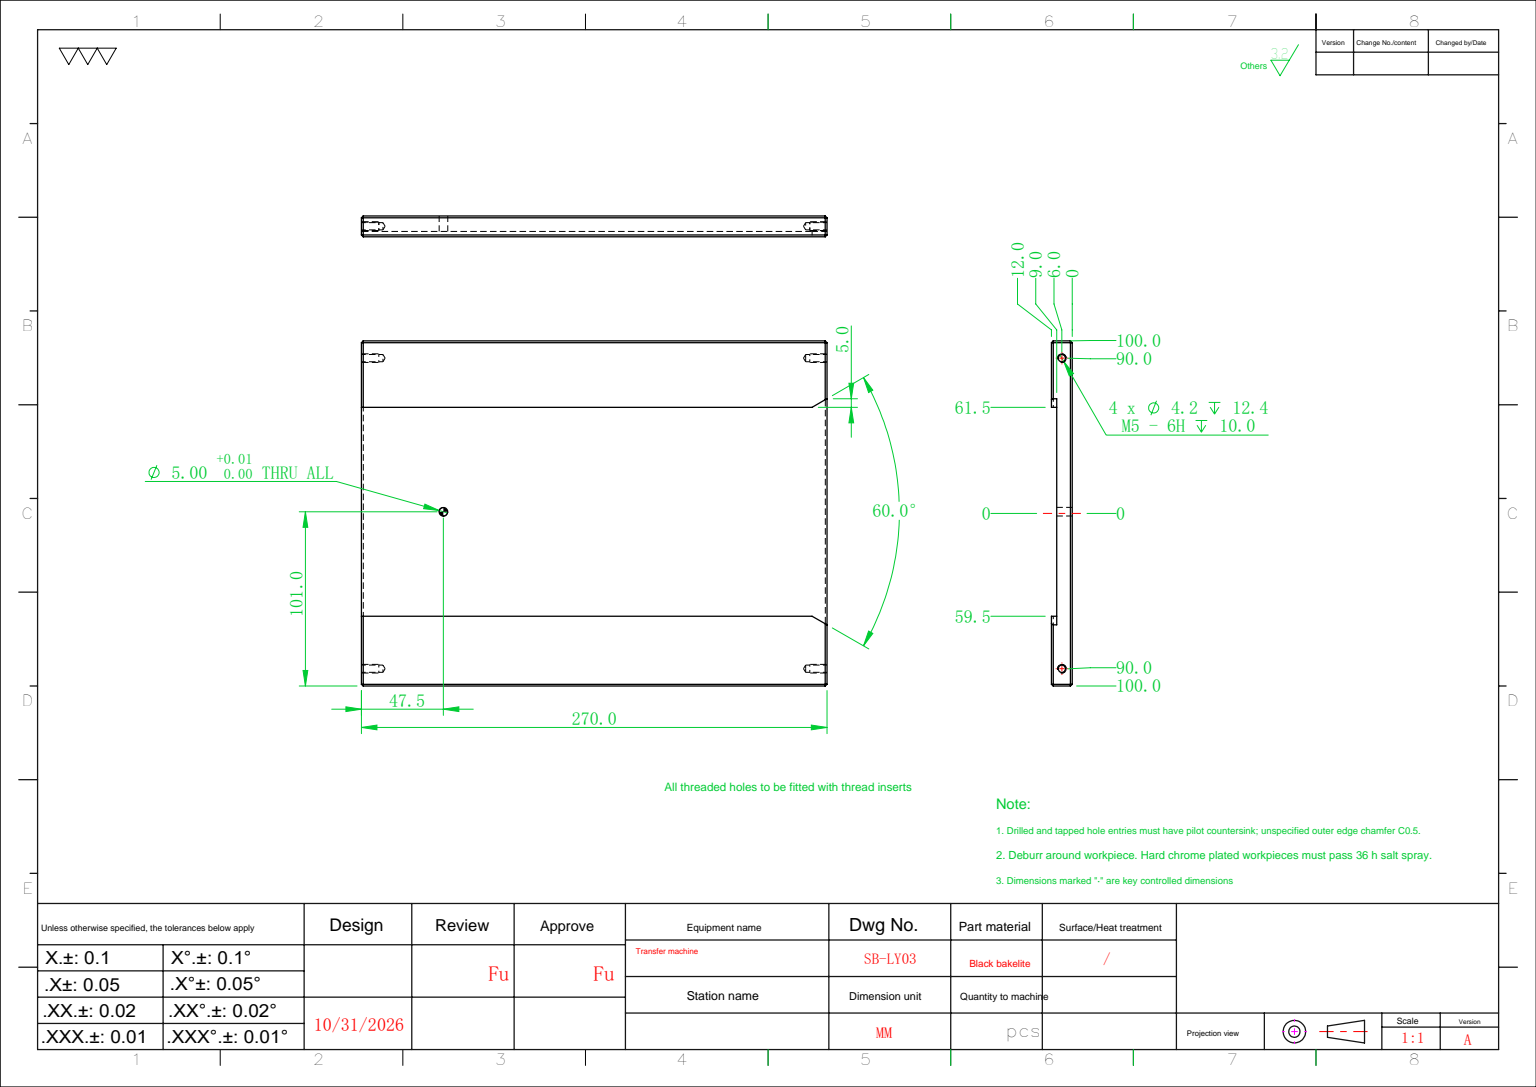
SolidWorks part; units mm, degrees
ref_plane "前视基准面" through (0, 0, 0) normal (0, 0, 1) x (1, 0, 0)
ref_plane "上视基准面" through (0, 0, 0) normal (0, 1, 0) x (1, 0, 0)
ref_plane "右视基准面" through (0, 0, 0) normal (1, 0, 0) x (0, 0, -1)
sketch "草图1" plane through (0, 0, 0) normal (0, 0, 1) x (1, 0, 0)
  line L1 (-100, -135) -> (100, -135)
  line L2 (-100, -135) -> (-100, 135)
  line L3 (-100, 135) -> (100, 135)
  line L4 (100, -135) -> (100, 135)
  line L5 (-100, -135) -> (100, 135) construction
  line L6 (-100, 135) -> (100, -135) construction
  point P0 (0, 0)
  dimension "D1" = 200
  dimension "D2" = 270
extrude "凸台-拉伸1" add sketch "草图1" along normal blind 12
sketch "草图2" plane through (0, 0, 12) normal (0, 0, 1) x (1, 0, 0)
  line L0 (100, 135) -> (-100, 135) construction
  line L1 (59.5, 135) -> (-61.5, 135)
  line L2 (59.5, 135) -> (59.5, -135)
  line L3 (59.5, -135) -> (-61.5, -135)
  line L4 (-61.5, 135) -> (-61.5, -135)
  line L5 (-100, -135) -> (100, -135) construction
  line L6 (-61, -82.7929) -> (-61, 147.7929) construction
  line L7 (59, 147.7929) -> (59, -82.7929) construction
  dimension "D1" = 0.5
  dimension "D2" = 0.5
extrude "切除-拉伸1" cut sketch "草图2" against normal blind 3
chamfer "倒角1" distance 5 angle 60 2 edges at (59.5, 135, 10.5) (-61.5, 135, 10.5)
hole_wizard "M5 螺纹孔1" positions "草图3" profile "草图4" tap size "M5" standard "ISO"
sketch "草图3" plane through (0, 135, 0) normal (0, 1, 0) x (1, 0, 0)
  line L0 (0, 0) -> (0, -9) construction
  line L1 (64.5, -9) -> (-66.5, -9) construction
  line L3 (100, -6) -> (-100, -6) construction
  line L4 (100, -12) -> (100, 0) construction
  line L5 (-100, -12) -> (-100, 0) construction
  point P0 (90, -6)
  point P2 (-90, -6)
  dimension "D1" = 180
sketch "草图4" plane through (90, 135, 6) normal (1, 0, 0) x (0, 0, 1)
  line L0 (0, 0) -> (0, 13.6618)
  line L1 (0, 13.6618) -> (2.1, 12.4)
  line L2 (2.1, 12.4) -> (2.1, 0)
  line L5 (2.1, 0) -> (0, 0)
  line L10 (0, 13.6618) -> (-2.1, 12.4) construction
  line L11 (0, -6.35) -> (0, 107.95) construction
  dimension "螺纹孔钻头直径" = 4.2
  dimension "螺纹孔钻头深度" = 12.4
  dimension "导头角度" = 118
cosmetic thread "孔螺蚊线1" parameters "D1"=10, "D2"=5
cosmetic thread "孔螺蚊线2" parameters "D1"=10, "D2"=5
mirror "镜向1" about plane through (0, 0, 0) normal (0, 1, 0) of "M5 螺纹孔1"
chamfer "倒角2" distance 1 angle 45 14 edges at (100, -135, 6) (79.75, -135, 12) (100, 0, 12) (82.25, 135, 12) (100, 135, 6) (100, 0, 0) (-100, 135, 6) (0, 135, 0) (-100, 0, 0) (0, -135, 0) (-100, -135, 6) (-80.75, -135, 12) (-100, 0, 12) (-83.25, 135, 12)
hole_wizard "大小mm 暗销孔1" positions "草图5" profile "草图6" hole size "Ø5.0" standard "ISO" end condition through all
sketch "草图5" plane through (0, 0, 9) normal (0, 0, 1) x (1, 0, 0)
  line L0 (-1, -135) -> (-1, -62.77) construction
  line L1 (-61.5, -135) -> (59.5, -135) construction
  point P0 (-1, -87.5)
  dimension "D1" = 47.5
sketch "草图6" plane through (-1, -87.5, 9) normal (1, 0, 0) x (0, -1, 0)
  line L0 (0, 0) -> (0, 9)
  line L1 (0, 9) -> (2.5, 9)
  line L2 (2.5, 9) -> (2.5, 0)
  line L5 (2.5, 0) -> (0, 0)
  line L11 (0, -6.35) -> (0, 107.95) construction
  dimension "通孔孔直径" = 5
  dimension "通孔孔深度" = 9
